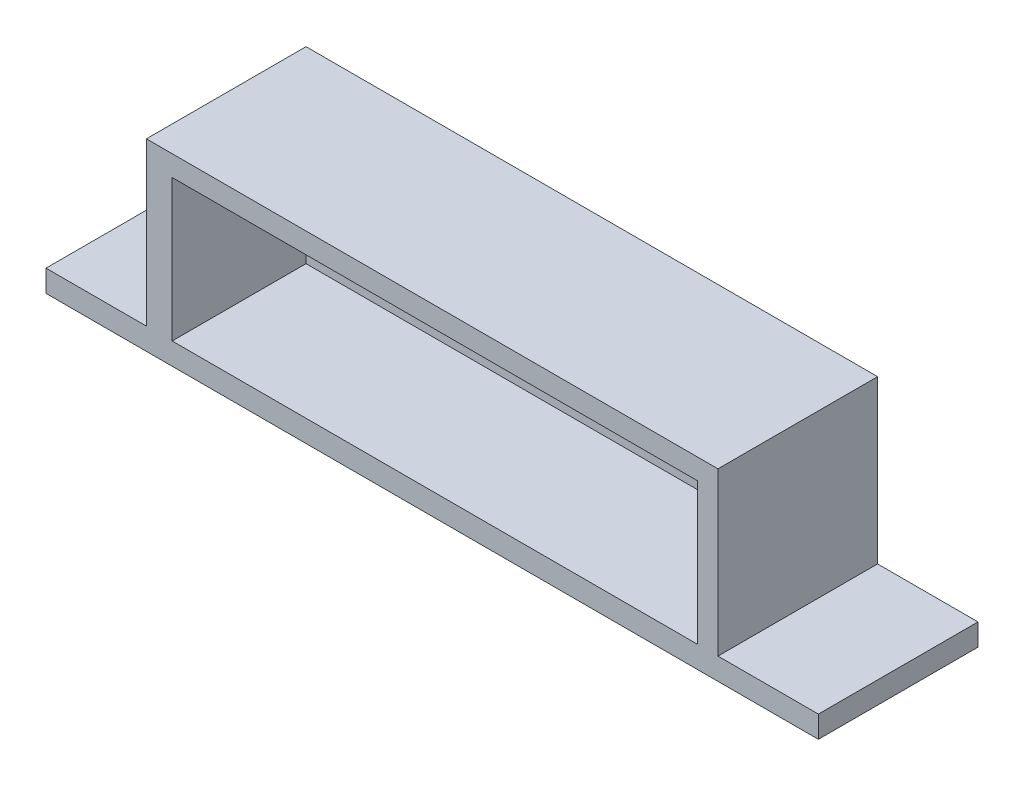
from build123d import *

# Parameters (mm, degrees)
SKETCH_1_W          = 300
SKETCH_1_H          = 62
EXTRUDE_1_DEPTH     = 5
SKETCH_2_W          = 298.120909486
SKETCH_2_H          = 12
CUT_EXTRUDE_1_DEPTH = 1.5
SKETCH_3_W          = 15
SKETCH_3_H          = 62
SKETCH_3_W_2        = 14
CUT_EXTRUDE_2_DEPTH = 1.5
EXTRUDE_2_DEPTH     = 55
SKETCH_5_W          = 222
SKETCH_5_H          = 62
EXTRUDE_3_DEPTH     = 8
CUT_EXTRUDE_3_REACH = 174.708
SKETCH_6_W          = 41.333333333
SKETCH_6_H          = 27
SKETCH_6_W_2        = 41.333333334
FILLET_1_R          = 5


with BuildPart() as part:
    # 草图1 → 凸台-拉伸1 (new, symmetric)
    with BuildSketch(Plane(origin=(0, 0, 0), x_dir=(1, 0, 0), z_dir=(0, 1, 0))):
        Rectangle(SKETCH_1_W, SKETCH_1_H)
    extrude(amount=EXTRUDE_1_DEPTH, both=True)

    # 草图2 → 切除-拉伸1 (cut)
    with BuildSketch(Plane.XZ.offset(5)):
        with Locations((0.939545257, 25)):
            Rectangle(SKETCH_2_W, SKETCH_2_H)
    extrude(amount=-CUT_EXTRUDE_1_DEPTH, mode=Mode.SUBTRACT)

    # 草图3 → 切除-拉伸2 (cut)
    with BuildSketch(Plane.XZ.offset(5)):
        with Locations((-142.5, 0)):
            Rectangle(SKETCH_3_W, SKETCH_3_H)
        with Locations((143, 0)):
            Rectangle(SKETCH_3_W_2, SKETCH_3_H)
    extrude(amount=-CUT_EXTRUDE_2_DEPTH, mode=Mode.SUBTRACT)

    # 草图4 → 凸台-拉伸2 (add)
    with BuildSketch(Plane(origin=(0, 5, 0), x_dir=(1, 0, 0), z_dir=(0, 1, 0))):
        Polygon((-111, -31), (-111, 31), (111, 31), (111, -31), (103, -31), (103, 21), (-101, 21), (-101, -31), align=None)
    extrude(amount=EXTRUDE_2_DEPTH)

    # 草图5 → 凸台-拉伸3 (add)
    with BuildSketch(Plane(origin=(0, 60, 0), x_dir=(1, 0, 0), z_dir=(0, 1, 0))):
        Rectangle(SKETCH_5_W, SKETCH_5_H)
    extrude(amount=EXTRUDE_3_DEPTH)

    # 草图6 → 切除-拉伸3 (cut, up to next)
    with BuildSketch(Plane.XY.offset(-21), mode=Mode.PRIVATE) as cut_extrude_3_sk1:
        with Locations((-60.333333334, 32.5)):
            Rectangle(SKETCH_6_W, SKETCH_6_H)
    cut_extrude_3_tool1 = extrude(cut_extrude_3_sk1.sketch, amount=-CUT_EXTRUDE_3_REACH, mode=Mode.PRIVATE) & part.part
    # 草图6 → 切除-拉伸3 (cut, up to next)
    with BuildSketch(Plane.XY.offset(-21), mode=Mode.PRIVATE) as cut_extrude_3_sk2:
        with Locations((62.333333334, 32.5)):
            Rectangle(SKETCH_6_W, SKETCH_6_H)
    cut_extrude_3_tool2 = extrude(cut_extrude_3_sk2.sketch, amount=-CUT_EXTRUDE_3_REACH, mode=Mode.PRIVATE) & part.part
    # 草图6 → 切除-拉伸3 (cut, up to next)
    with BuildSketch(Plane.XY.offset(-21), mode=Mode.PRIVATE) as cut_extrude_3_sk3:
        with Locations((1, 32.5)):
            Rectangle(SKETCH_6_W_2, SKETCH_6_H)
    cut_extrude_3_tool3 = extrude(cut_extrude_3_sk3.sketch, amount=-CUT_EXTRUDE_3_REACH, mode=Mode.PRIVATE) & part.part
    add(cut_extrude_3_tool1.solids().sort_by_distance((-60.333333, 32.5, -21))[0], mode=Mode.SUBTRACT)
    add(cut_extrude_3_tool2.solids().sort_by_distance((62.333333, 32.5, -21))[0], mode=Mode.SUBTRACT)
    add(cut_extrude_3_tool3.solids().sort_by_distance((1, 32.5, -21))[0], mode=Mode.SUBTRACT)

    # 圆角1
    fillet_1_edges = [part.edges().sort_by_distance(p)[0] for p in [
        (-39.666666667, 46, -26),
        (-39.666666667, 19, -26),
        (-81, 19, -26),
        (-81, 46, -26),
        (83, 46, -26),
        (83, 19, -26),
        (41.666666667, 19, -26),
        (41.666666667, 46, -26),
        (21.666666667, 46, -26),
        (21.666666667, 19, -26),
        (-19.666666667, 19, -26),
        (-19.666666667, 46, -26),
    ]]
    fillet(fillet_1_edges, radius=FILLET_1_R)


solid = part.part
